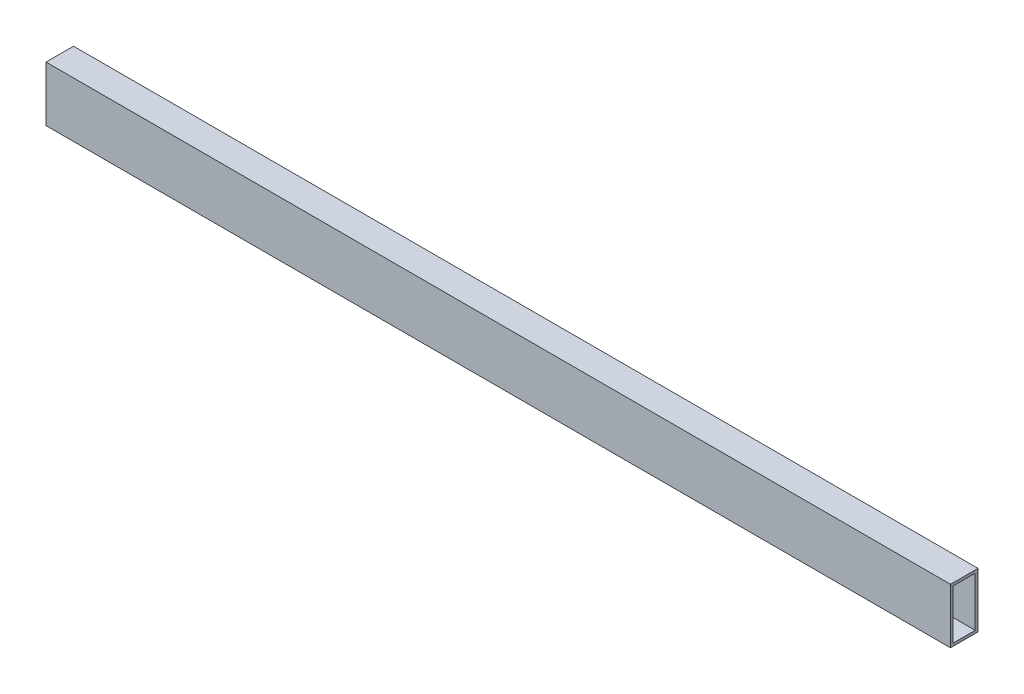
SolidWorks part; units mm, degrees
ref_plane "Front Plane" through (0, 0, 0) normal (0, 0, 1) x (1, 0, 0)
ref_plane "Top Plane" through (0, 0, 0) normal (0, 1, 0) x (1, 0, 0)
ref_plane "Right Plane" through (0, 0, 0) normal (1, 0, 0) x (0, 0, -1)
sketch "Sketch1" plane through (0, 0, 0) normal (0, 0, 1) x (1, 0, 0)
  line L0 (473, -13) -> (473, 13) construction
  line L1 (-493, 30) -> (493, 30)
  line L2 (-493, 30) -> (-493, -30)
  line L3 (-493, -30) -> (493, -30)
  line L4 (493, 30) -> (493, -30)
  line L5 (-493, 30) -> (493, -30) construction
  line L6 (-493, -30) -> (493, 30) construction
  point P0 (0, 0)
  dimension "D1" = 20
  dimension "D2" = 60
extrude "Boss-Extrude1" add sketch "Sketch1" along normal blind 30
sketch "Sketch2" plane through (-493, 0, 0) normal (-1, 0, 0) x (0, 0, 1)
  line L8 (3, 27) -> (3, -27)
  line L9 (3, -27) -> (27, -27)
  line L10 (27, -27) -> (27, 27)
  line L11 (27, 27) -> (3, 27)
  line L12 (3, 27) -> (3, -27)
  line L13 (3, -27) -> (27, -27)
  line L14 (27, -27) -> (27, 27)
  line L15 (27, 27) -> (3, 27)
  dimension "D1" = 3
extrude "Cut-Extrude1" cut sketch "Sketch2" against normal blind 2043
